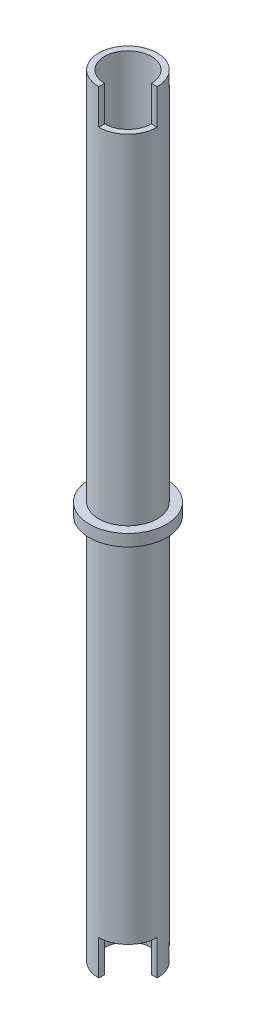
SolidWorks part; units mm, degrees
ref_plane "Front Plane" through (0, 0, 0) normal (0, 0, 1) x (1, 0, 0)
ref_plane "Top Plane" through (0, 0, 0) normal (0, 1, 0) x (1, 0, 0)
ref_plane "Right Plane" through (0, 0, 0) normal (1, 0, 0) x (0, 0, -1)
sketch "Sketch1" plane through (0, 0, 0) normal (0, 0, 1) x (1, 0, 0)
  line L0 (0, 0) -> (25, 0)
  line L1 (25, 0) -> (25, 330)
  line L2 (25, 330) -> (33, 330)
  line L3 (33, 330) -> (33, 340)
  line L4 (33, 340) -> (25, 340)
  line L5 (25, 340) -> (25, 585.1197)
  line L9 (25, 585.1197) -> (25, 619.0324)
  line L13 (25, 619.0324) -> (25, 660)
  line L14 (25, 660) -> (0, 660)
  line L15 (0, 660) -> (0, 0)
  dimension "D1" = 25
  dimension "D2" = 25
  dimension "D5" = 340
  dimension "D6" = 8
  dimension "D7" = 10
  dimension "D10" = 660
revolve "Revolve1" add sketch "Sketch1" angle 360 about L15
sketch "Sketch2" plane through (0, 660, 0) normal (0, 1, 0) x (1, 0, 0)
  circle A0 centre (0, 0) radius 20
  dimension "D1" = 40
extrude "Cut-Extrude1" cut sketch "Sketch2" against normal up to next
sketch "Sketch3" plane through (0, 660, 0) normal (0, 1, 0) x (1, 0, 0)
  line L0 (0, -43.2015) -> (0, 0)
  line L1 (0, 0) -> (43.2015, 0)
  arc A0 (43.2015, 0) -> (0, -43.2015) centre (0, 0) cw
extrude "Cut-Extrude2" cut sketch "Sketch3" against normal blind 30
sketch "Sketch4" plane through (0, 0, 0) normal (0, -1, 0) x (1, 0, 0)
  line L0 (51.0682, 0) -> (0, 0)
  line L1 (0, 0) -> (0, 51.0682)
  arc A0 (51.0682, 0) -> (0, 51.0682) centre (0, 0) ccw
extrude "Cut-Extrude3" cut sketch "Sketch4" against normal blind 30
